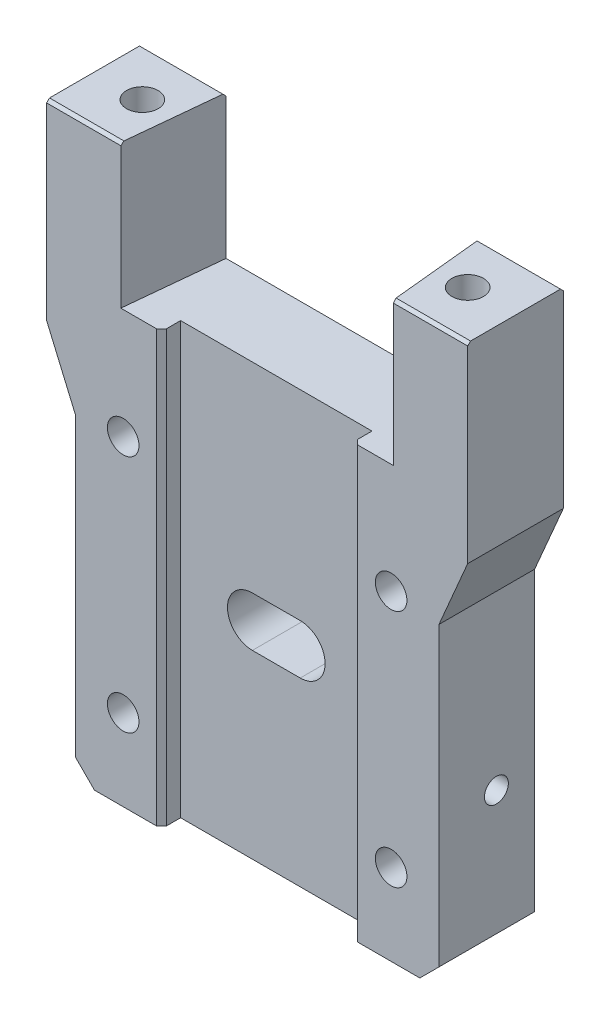
SolidWorks part; units mm, degrees
ref_plane "Front Plane" through (0, 0, 0) normal (0, 0, 1) x (1, 0, 0)
ref_plane "Top Plane" through (0, 0, 0) normal (0, 1, 0) x (1, 0, 0)
ref_plane "Right Plane" through (0, 0, 0) normal (1, 0, 0) x (0, 0, -1)
sketch "Sketch1" plane through (0, 0, 0) normal (0, 0, 1) x (1, 0, 0)
  line L1 (-22, -30) -> (22, -30)
  line L2 (-22, -30) -> (-22, 30)
  line L3 (-22, 30) -> (22, 30)
  line L4 (22, -30) -> (22, 30)
  line L5 (-22, -30) -> (22, 30) construction
  line L6 (-22, 30) -> (22, -30) construction
  point P0 (0, 0)
  dimension "D1" = 44
  dimension "D2" = 60
extrude "Boss-Extrude1" add sketch "Sketch1" along normal blind 10
sketch "Sketch13" plane through (0, 30, 0) normal (0, 1, 0) x (1, 0, 0)
  line L0 (13.25, 0) -> (14.25, -10)
  line L1 (22, 0) -> (-22, 0) construction
  line L2 (22, -10) -> (-22, -10) construction
  line L3 (14.25, -10) -> (-14.25, -10)
  line L4 (-14.25, -10) -> (-13.25, 0)
  line L5 (-13.25, 0) -> (13.25, 0)
  line L6 (0, 0) -> (0, -16.8561) construction
  dimension "D1" = 26.5
  dimension "D2" = 28.5
extrude "Cut-Extrude4" cut sketch "Sketch13" against normal blind 15
sketch "Sketch2" plane through (0, 0, 10) normal (0, 0, 1) x (1, 0, 0)
  line L1 (10, -30) -> (-10, -30)
  line L2 (10, -30) -> (10, 30)
  line L3 (10, 30) -> (-10, 30)
  line L4 (-10, -30) -> (-10, 30)
  line L7 (22, 30) -> (14.25, 30) construction
  line L8 (-22, -30) -> (22, -30) construction
  line L9 (0, 0) -> (0, 12.0004) construction
  point P0 (0, 0)
  dimension "D1" = 20
extrude "Cut-Extrude1" cut sketch "Sketch2" against normal blind 2
hole_wizard "M4 Tapped Hole1" positions "Sketch4" profile "Sketch3" tap size "M4" standard "Gb"
sketch "Sketch4" plane through (0, 30, 0) normal (0, 1, 0) x (1, 0, 0)
  line L5 (-22, -5) -> (22, -5) construction
  line L8 (22, 0) -> (13.25, 0) construction
  line L9 (0, 0) -> (0, -6.1264) construction
  line L10 (13.25, 0) -> (-13.25, 0) construction
  point P0 (-17, -5)
  point P2 (17, -5)
  dimension "D1" = 34
  dimension "D2" = 5
sketch "Sketch3" plane through (-17, 30, 5) normal (1, 0, 0) x (0, 0, 1)
  line L0 (0, 0) -> (0, 11.0914)
  line L1 (0, 11.0914) -> (1.65, 10.1)
  line L2 (1.65, 10.1) -> (1.65, 0)
  line L5 (1.65, 0) -> (0, 0)
  line L10 (0, 11.0914) -> (-1.65, 10.1) construction
  line L11 (0, -6.35) -> (0, 107.95) construction
  dimension "螺纹孔钻头直径" = 3.3
  dimension "螺纹孔钻头深度" = 10.1
  dimension "导头角度" = 118
cosmetic thread "Hole thread 11" parameters "D1"=8, "D2"=4
cosmetic thread "Hole thread 12" parameters "D1"=8, "D2"=4
hole_wizard "M4 Tapped Hole2" positions "Sketch6" profile "Sketch5" tap size "M4" standard "Gb"
sketch "Sketch6" plane through (0, 0, 10) normal (0, 0, 1) x (1, 0, 0)
  line L1 (0, 0) -> (0, -19.7946) construction
  line L3 (10, -30) -> (22, -30) construction
  point P0 (-14, -21.5)
  point P2 (14, -21.5)
  point P4 (-14, 3.5)
  point P6 (14, 3.5)
  dimension "D1" = 8.5
  dimension "D2" = 25
  dimension "D3" = 28
sketch "Sketch5" plane through (-14, -21.5, 10) normal (1, 0, 0) x (0, -1, 0)
  line L0 (0, 0) -> (0, 11.0914)
  line L1 (0, 11.0914) -> (1.65, 10.1)
  line L2 (1.65, 10.1) -> (1.65, 0)
  line L5 (1.65, 0) -> (0, 0)
  line L10 (0, 11.0914) -> (-1.65, 10.1) construction
  line L11 (0, -6.35) -> (0, 107.95) construction
  dimension "螺纹孔钻头直径" = 3.3
  dimension "螺纹孔钻头深度" = 10.1
  dimension "导头角度" = 118
cosmetic thread "Hole thread 3" parameters "D1"=8, "D2"=4
cosmetic thread "Hole thread 4" parameters "D1"=8, "D2"=4
cosmetic thread "Hole thread 5" parameters "D1"=8, "D2"=4
cosmetic thread "Hole thread 6" parameters "D1"=8, "D2"=4
hole_wizard "M3 Tapped Hole2" positions "Sketch10" profile "Sketch9" tap size "M3" standard "Gb"
sketch "Sketch10" plane through (22, 0, 0) normal (1, 0, 0) x (0, 0, -1)
  line L0 (-10, -30) -> (0, -30) construction
  line L1 (0, -30) -> (0, 30) construction
  point P0 (-4, -15)
  dimension "D1" = 15
  dimension "D2" = 4
sketch "Sketch9" plane through (22, -15, 4) normal (0, 1, 0) x (0, 0, -1)
  line L0 (0, 0) -> (0, 8.2511)
  line L1 (0, 8.2511) -> (1.25, 7.5)
  line L2 (1.25, 7.5) -> (1.25, 0)
  line L5 (1.25, 0) -> (0, 0)
  line L10 (0, 8.2511) -> (-1.25, 7.5) construction
  line L11 (0, -6.35) -> (0, 107.95) construction
  dimension "螺纹孔钻头直径" = 2.5
  dimension "螺纹孔钻头深度" = 7.5
  dimension "导头角度" = 118
cosmetic thread "Hole thread 9" parameters "D1"=6, "D2"=3
sketch "Sketch11" plane through (22, 0, 0) normal (1, 0, 0) x (0, 0, -1)
  line L1 (-10, 30) -> (-9, 30)
  line L2 (-10, 30) -> (-10, 28.8)
  line L3 (-10, 28.8) -> (-9, 28.8)
  line L4 (-9, 30) -> (-9, 28.8)
  dimension "D1" = 1.2
  dimension "D2" = 1
extrude "Cut-Extrude2" [suppressed] cut sketch "Sketch11" against normal through all
chamfer "Chamfer3" distance 0.3 angle 45 4 edges at (17.625, 30, 0) (-17.625, 30, 0) (-18.125, 30, 10) (18.125, 30, 10)
chamfer "Chamfer4" distance 0.5 angle 45 2 edges at (10, -7.5, 10) (-10, -7.5, 10)
sketch "Sketch14" plane through (0, 0, 10) normal (0, 0, 1) x (1, 0, 0)
  line L0 (-19, -30) -> (-19, 3)
  line L1 (-22, -30) -> (-10.5, -30) construction
  line L2 (-19, 3) -> (-22, 10)
  line L3 (-22, 29.7) -> (-22, -30) construction
  line L4 (-22, 10) -> (-22, -30)
  line L5 (-22, -30) -> (-19, -30)
  line L6 (19, -30) -> (19, 3)
  line L7 (10.5, -30) -> (22, -30) construction
  line L8 (19, 3) -> (22, 10)
  line L9 (22, -30) -> (22, 29.7) construction
  line L10 (22, 10) -> (22, -30)
  line L11 (22, -30) -> (19, -30)
  line L12 (0, 0) -> (0, -38.4893) construction
  dimension "D1" = 38
  dimension "D2" = 40
  dimension "D3" = 33
extrude "Cut-Extrude5" cut sketch "Sketch14" against normal through all
chamfer "Chamfer5" distance 2 angle 45 2 edges at (19, -30, 5) (-19, -30, 5)
sketch "Sketch15" plane through (0, 0, 0) normal (0, 0, -1) x (-1, 0, 0)
  line L0 (-2.5, -8.5) -> (2.5, -8.5) construction
  line L1 (-2.5, -5.9) -> (2.5, -5.9)
  line L2 (-2.5, -11.1) -> (2.5, -11.1)
  line L3 (17, -30) -> (-17, -30) construction
  line L4 (0, -30) -> (0, 3.0673) construction
  arc A0 (-2.5, -5.9) -> (-2.5, -11.1) centre (-2.5, -8.5) ccw
  arc A1 (2.5, -11.1) -> (2.5, -5.9) centre (2.5, -8.5) ccw
  point P2 (0, -8.5)
  dimension "D1" = 21.5
  dimension "D2" = 5
  dimension "D3" = 5.2
extrude "Cut-Extrude6" cut sketch "Sketch15" against normal through all
